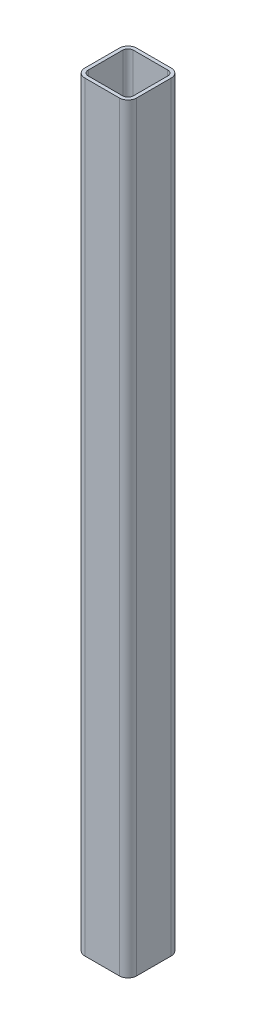
SolidWorks part; units mm, degrees
material "Q235B"
ref_plane "Front Plane" through (0, 0, 0) normal (0, 0, 1) x (1, 0, 0)
ref_plane "Top Plane" through (0, 0, 0) normal (0, 1, 0) x (1, 0, 0)
ref_plane "Right Plane" through (0, 0, 0) normal (1, 0, 0) x (0, 0, -1)
other "Configuration Table"
sketch "Sketch1" plane through (0, 0, 0) normal (0, 1, 0) x (1, 0, 0)
  line L0 (-26, -20) -> (-26, 20)
  line L1 (-20, -30) -> (20, -30)
  line L2 (-30, -20) -> (-30, 20)
  line L3 (-20, 30) -> (20, 30)
  line L4 (30, -20) -> (30, 20)
  line L5 (-30, -30) -> (30, 30) construction
  line L6 (-30, 30) -> (30, -30) construction
  line L7 (-20, 26) -> (20, 26)
  line L8 (26, -20) -> (26, 20)
  line L9 (-20, -26) -> (20, -26)
  arc A0 (20, -30) -> (30, -20) centre (20, -20) ccw
  arc A1 (-20, -30) -> (-30, -20) centre (-20, -20) cw
  arc A2 (20, 30) -> (30, 20) centre (20, 20) cw
  arc A3 (-30, 20) -> (-20, 30) centre (-20, 20) cw
  arc A4 (-26, 20) -> (-20, 26) centre (-20, 20) cw
  arc A5 (20, 26) -> (26, 20) centre (20, 20) cw
  arc A6 (20, -26) -> (26, -20) centre (20, -20) ccw
  arc A7 (-20, -26) -> (-26, -20) centre (-20, -20) cw
  point P0 (0, 0)
  dimension "D2" = 10
  dimension "D1" = 60
  dimension "D3" = 4
extrude "Boss-Extrude1" add sketch "Sketch1" along normal blind 880
